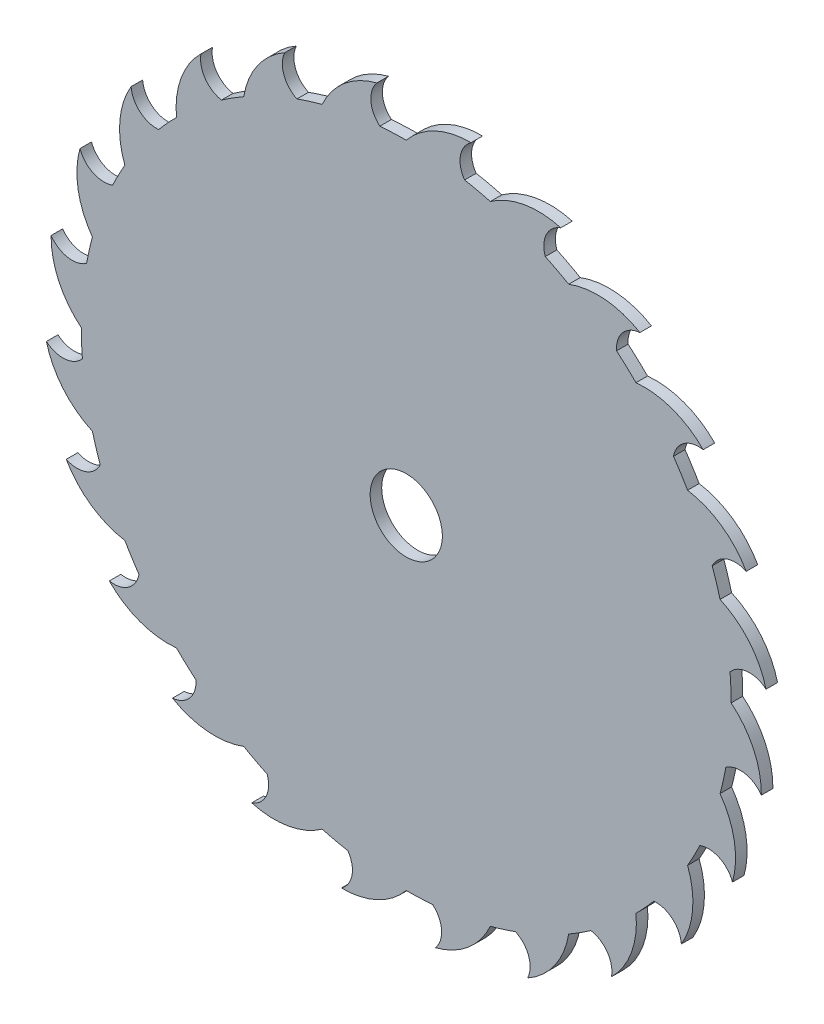
from build123d import *

# Parameters (mm, degrees)
SKETCH1_R           = 12.5
BOSS_EXTRUDE1_DEPTH = 4


with BuildPart() as part:
    # Sketch1 → Boss-Extrude1 (new body)
    with BuildSketch(Plane.XY.offset(4)):
        with BuildLine():
            ThreePointArc((22.440452668, 122.96920787), (10.028572641, 120.288880116), (0, 112.5))
            ThreePointArc((0, 112.5), (-4.571708495, 112.407070425), (-9.135864155, 112.128435226))
            ThreePointArc((-9.135864155, 112.128435226), (-12.223696531, 118.147559469), (-10.150960173, 124.587150251))
            ThreePointArc((-10.150960173, 124.587150251), (-21.446195774, 118.785721514), (-29.117142574, 108.666655458))
            ThreePointArc((-29.117142574, 108.666655458), (-33.509021935, 107.393647153), (-37.845541667, 105.943215809))
            ThreePointArc((-37.845541667, 105.943215809), (-42.386022695, 110.958053541), (-42.050601852, 117.714684232))
            ThreePointArc((-42.050601852, 117.714684232), (-51.459441387, 109.187512293), (-56.25, 97.427857926))
            ThreePointArc((-56.25, 97.427857926), (-60.162750907, 95.061524305), (-63.976108057, 92.538141314))
            ThreePointArc((-63.976108057, 92.538141314), (-69.659811458, 96.20693963), (-71.084564508, 102.820157016))
            ThreePointArc((-71.084564508, 102.820157016), (-77.965811111, 92.148354551), (-79.549512883, 79.549512883))
            ThreePointArc((-79.549512883, 79.549512883), (-82.716487829, 76.251115672), (-85.746808408, 72.826745416))
            ThreePointArc((-85.746808408, 72.826745416), (-92.186399189, 74.899481774), (-95.274231565, 80.918606017))
            ThreePointArc((-95.274231565, 80.918606017), (-99.158939653, 68.829438728), (-97.427857926, 56.25))
            ThreePointArc((-97.427857926, 56.25), (-99.6332328, 52.244319517), (-101.67400547, 48.152327169))
            ThreePointArc((-101.67400547, 48.152327169), (-108.430636161, 48.487748011), (-112.971117188, 53.502585743))
            ThreePointArc((-112.971117188, 53.502585743), (-113.594550325, 40.819910403), (-108.666655458, 29.117142574))
            ThreePointArc((-108.666655458, 29.117142574), (-109.760137608, 24.677159325), (-110.672287083, 20.196407401))
            ThreePointArc((-110.672287083, 20.196407401), (-117.285504468, 18.771654352), (-122.96920787, 22.440452668))
            ThreePointArc((-122.96920787, 22.440452668), (-120.288880116, 10.028572641), (-112.5, 0))
            ThreePointArc((-112.5, 0), (-112.407070425, -4.571708495), (-112.128435226, -9.135864155))
            ThreePointArc((-112.128435226, -9.135864155), (-118.147559469, -12.223696531), (-124.587150251, -10.150960173))
            ThreePointArc((-124.587150251, -10.150960173), (-118.785721514, -21.446195774), (-108.666655458, -29.117142574))
            ThreePointArc((-108.666655458, -29.117142574), (-107.393647153, -33.509021935), (-105.943215809, -37.845541667))
            ThreePointArc((-105.943215809, -37.845541667), (-110.958053541, -42.386022695), (-117.714684232, -42.050601852))
            ThreePointArc((-117.714684232, -42.050601852), (-109.187512293, -51.459441387), (-97.427857926, -56.25))
            ThreePointArc((-97.427857926, -56.25), (-95.061524305, -60.162750907), (-92.538141314, -63.976108057))
            ThreePointArc((-92.538141314, -63.976108057), (-96.20693963, -69.659811458), (-102.820157016, -71.084564508))
            ThreePointArc((-102.820157016, -71.084564508), (-92.148354551, -77.965811111), (-79.549512883, -79.549512883))
            ThreePointArc((-79.549512883, -79.549512883), (-76.251115672, -82.716487829), (-72.826745416, -85.746808408))
            ThreePointArc((-72.826745416, -85.746808408), (-74.899481774, -92.186399189), (-80.918606017, -95.274231565))
            ThreePointArc((-80.918606017, -95.274231565), (-68.829438728, -99.158939653), (-56.25, -97.427857926))
            ThreePointArc((-56.25, -97.427857926), (-52.244319517, -99.6332328), (-48.152327169, -101.67400547))
            ThreePointArc((-48.152327169, -101.67400547), (-48.487748011, -108.430636161), (-53.502585743, -112.971117188))
            ThreePointArc((-53.502585743, -112.971117188), (-40.819910403, -113.594550325), (-29.117142574, -108.666655458))
            ThreePointArc((-29.117142574, -108.666655458), (-24.677159325, -109.760137608), (-20.196407401, -110.672287083))
            ThreePointArc((-20.196407401, -110.672287083), (-18.771654352, -117.285504468), (-22.440452668, -122.96920787))
            ThreePointArc((-22.440452668, -122.96920787), (-10.028572641, -120.288880116), (0, -112.5))
            ThreePointArc((0, -112.5), (4.571708495, -112.407070425), (9.135864155, -112.128435226))
            ThreePointArc((9.135864155, -112.128435226), (12.223696531, -118.147559469), (10.150960173, -124.587150251))
            ThreePointArc((10.150960173, -124.587150251), (21.446195774, -118.785721514), (29.117142574, -108.666655458))
            ThreePointArc((29.117142574, -108.666655458), (33.509021935, -107.393647153), (37.845541667, -105.943215809))
            ThreePointArc((37.845541667, -105.943215809), (42.386022695, -110.958053541), (42.050601852, -117.714684232))
            ThreePointArc((42.050601852, -117.714684232), (51.459441387, -109.187512293), (56.25, -97.427857926))
            ThreePointArc((56.25, -97.427857926), (60.162750907, -95.061524305), (63.976108057, -92.538141314))
            ThreePointArc((63.976108057, -92.538141314), (69.659811458, -96.20693963), (71.084564508, -102.820157016))
            ThreePointArc((71.084564508, -102.820157016), (77.965811111, -92.148354551), (79.549512883, -79.549512883))
            ThreePointArc((79.549512883, -79.549512883), (82.716487829, -76.251115672), (85.746808408, -72.826745416))
            ThreePointArc((85.746808408, -72.826745416), (92.186399189, -74.899481774), (95.274231565, -80.918606017))
            ThreePointArc((95.274231565, -80.918606017), (99.158939653, -68.829438728), (97.427857926, -56.25))
            ThreePointArc((97.427857926, -56.25), (99.6332328, -52.244319517), (101.67400547, -48.152327169))
            ThreePointArc((101.67400547, -48.152327169), (108.430636161, -48.487748011), (112.971117188, -53.502585743))
            ThreePointArc((112.971117188, -53.502585743), (113.594550325, -40.819910403), (108.666655458, -29.117142574))
            ThreePointArc((108.666655458, -29.117142574), (109.760137608, -24.677159325), (110.672287083, -20.196407401))
            ThreePointArc((110.672287083, -20.196407401), (117.285504468, -18.771654352), (122.96920787, -22.440452668))
            ThreePointArc((122.96920787, -22.440452668), (120.288880116, -10.028572641), (112.5, 0))
            ThreePointArc((112.5, 0), (112.407070425, 4.571708495), (112.128435226, 9.135864155))
            ThreePointArc((112.128435226, 9.135864155), (118.147559469, 12.223696531), (124.587150251, 10.150960173))
            ThreePointArc((124.587150251, 10.150960173), (118.785721514, 21.446195774), (108.666655458, 29.117142574))
            ThreePointArc((108.666655458, 29.117142574), (107.393647153, 33.509021935), (105.943215809, 37.845541667))
            ThreePointArc((105.943215809, 37.845541667), (110.958053541, 42.386022695), (117.714684232, 42.050601852))
            ThreePointArc((117.714684232, 42.050601852), (109.187512293, 51.459441387), (97.427857926, 56.25))
            ThreePointArc((97.427857926, 56.25), (95.061524305, 60.162750907), (92.538141314, 63.976108057))
            ThreePointArc((92.538141314, 63.976108057), (96.20693963, 69.659811458), (102.820157016, 71.084564508))
            ThreePointArc((102.820157016, 71.084564508), (92.148354551, 77.965811111), (79.549512883, 79.549512883))
            ThreePointArc((79.549512883, 79.549512883), (76.251115672, 82.716487829), (72.826745416, 85.746808408))
            ThreePointArc((72.826745416, 85.746808408), (74.899481774, 92.186399189), (80.918606017, 95.274231565))
            ThreePointArc((80.918606017, 95.274231565), (68.829438728, 99.158939653), (56.25, 97.427857926))
            ThreePointArc((56.25, 97.427857926), (52.244319517, 99.6332328), (48.152327169, 101.67400547))
            ThreePointArc((48.152327169, 101.67400547), (48.487748011, 108.430636161), (53.502585743, 112.971117188))
            ThreePointArc((53.502585743, 112.971117188), (40.819910403, 113.594550325), (29.117142574, 108.666655458))
            ThreePointArc((29.117142574, 108.666655458), (24.677159325, 109.760137608), (20.196407401, 110.672287083))
            ThreePointArc((20.196407401, 110.672287083), (18.771654352, 117.285504468), (22.440452668, 122.96920787))
        make_face()
        with Locations(Location((0, 0, 0), (0, 0, 180))):
            Circle(SKETCH1_R, mode=Mode.SUBTRACT)
    extrude(amount=-BOSS_EXTRUDE1_DEPTH)


solid = part.part
